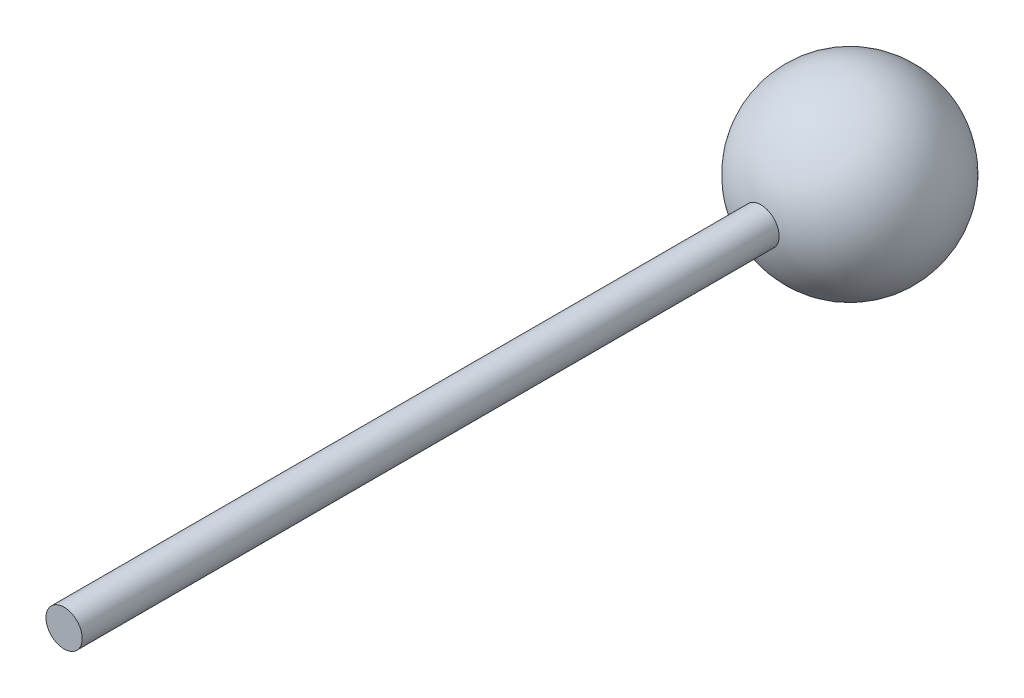
from build123d import *

# Parameters (mm, degrees)
SKETCH2_R           = 3
BOSS_EXTRUDE1_DEPTH = 130


with BuildPart() as part:
    # Sketch1 → Revolve3 (revolve)
    with BuildSketch(Plane(origin=(0, 0, 0), x_dir=(1, 0, 0), z_dir=(0, 1, 0))):
        with BuildLine():
            Line((0, 15), (0, -15))
            ThreePointArc((0, -15), (-15, 0), (0, 15))
        make_face()
    revolve(axis=Axis((0, 0, 1000), (0, 0, -1)))

    # Sketch2 → Boss-Extrude1 (add)
    with BuildSketch(Plane.XY):
        Circle(SKETCH2_R)
    extrude(amount=BOSS_EXTRUDE1_DEPTH)


solid = part.part
